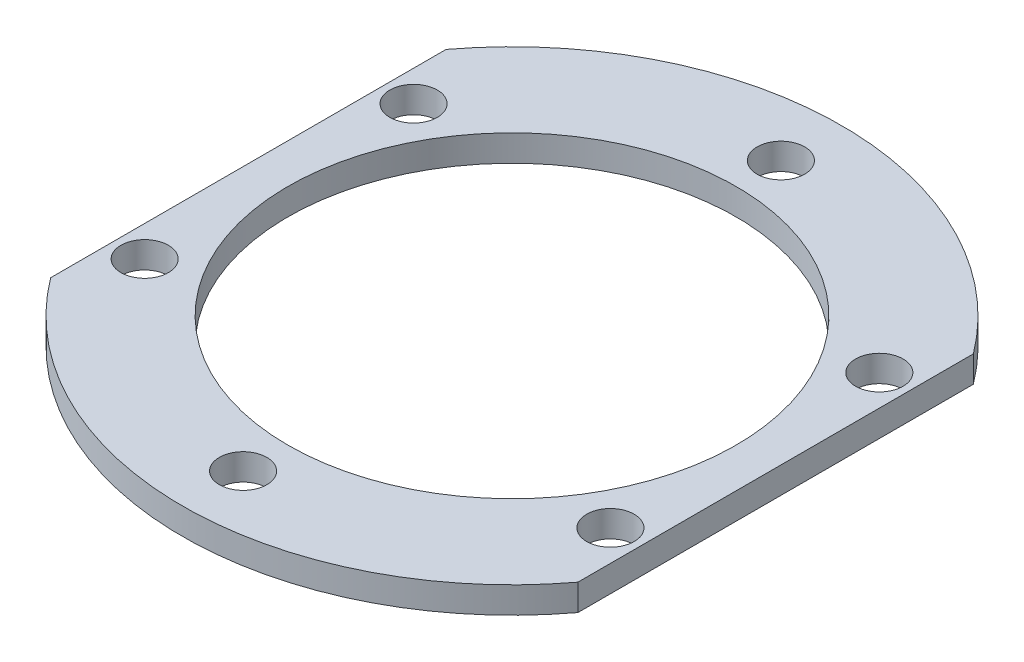
SolidWorks part; units mm, degrees
material "普通碳钢"
ref_plane "Front Plane" through (0, 0, 0) normal (0, 0, 1) x (1, 0, 0)
ref_plane "Top Plane" through (0, 0, 0) normal (0, 1, 0) x (1, 0, 0)
ref_plane "Right Plane" through (0, 0, 0) normal (1, 0, 0) x (0, 0, -1)
sketch "Sketch1" plane through (0, 0, 0) normal (0, 1, 0) x (1, 0, 0)
  circle A0 centre (0, 0) radius 62.5
  circle A1 centre (0, 0) radius 42.5
  dimension "D1" = 125
  dimension "D2" = 85
extrude "Boss-Extrude1" add sketch "Sketch1" along normal blind 5
sketch "Sketch2" plane through (0, 5, 0) normal (0, 1, 0) x (1, 0, 0)
  circle A0 centre (0, 0) radius 51 construction
  circle A1 centre (0, 51) radius 4.5
  circle A2 centre (44.1673, 25.5) radius 4.5
  circle A3 centre (44.1673, -25.5) radius 4.5
  circle A4 centre (0, -51) radius 4.5
  circle A5 centre (-44.1673, -25.5) radius 4.5
  circle A6 centre (-44.1673, 25.5) radius 4.5
  point P17 (0, 0)
  dimension "D1" = 102
  dimension "D2" = 9
  dimension "D3" = 6
extrude "Cut-Extrude1" cut sketch "Sketch2" against normal blind 10
sketch "Sketch3" plane through (0, 5, 0) normal (0, 1, 0) x (1, 0, 0)
  line L1 (50, -71.7656) -> (-50, -71.7656)
  line L2 (50, -71.7656) -> (50, 71.7656)
  line L3 (50, 71.7656) -> (-50, 71.7656)
  line L4 (-50, -71.7656) -> (-50, 71.7656)
  line L5 (50, -71.7656) -> (-50, 71.7656) construction
  line L6 (50, 71.7656) -> (-50, -71.7656) construction
  point P0 (0, 0)
  dimension "D1" = 100
  dimension "D2" = 143.5312
extrude "Cut-Extrude2" cut sketch "Sketch3" against normal blind 10 flip side to cut
